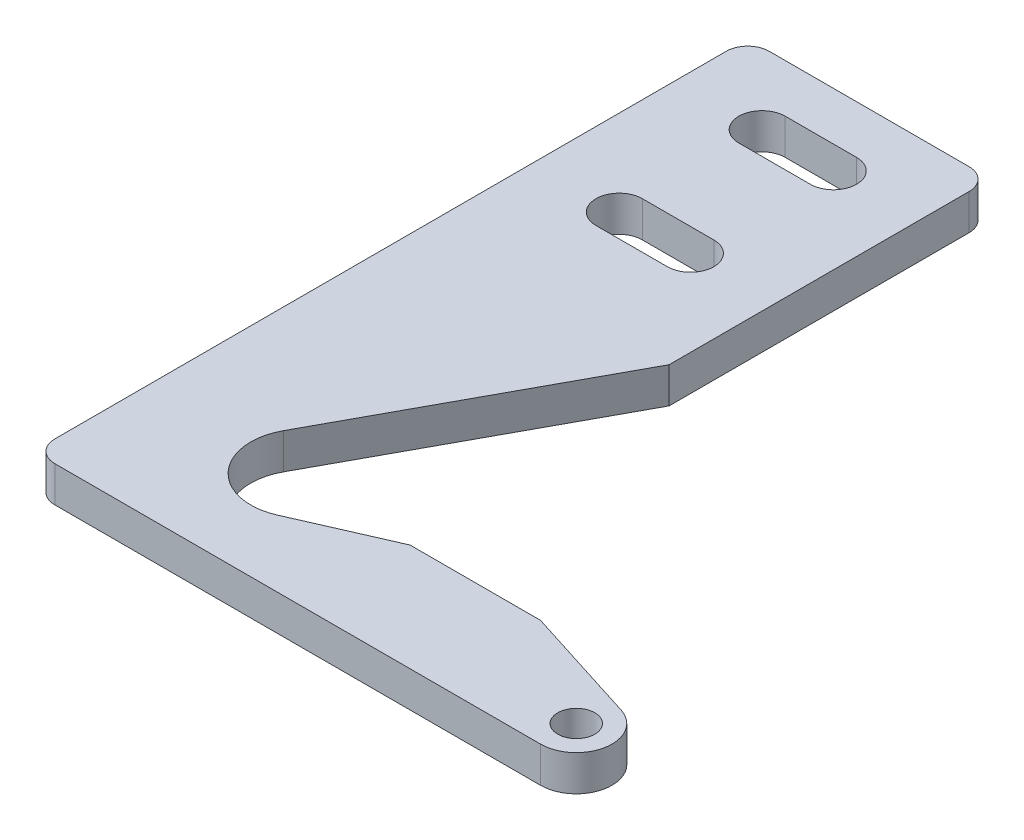
SolidWorks part; units mm, degrees
material "SPCC"
ref_plane "Front Plane" through (0, 0, 0) normal (0, 0, 1) x (1, 0, 0)
ref_plane "Top Plane" through (0, 0, 0) normal (0, 1, 0) x (1, 0, 0)
ref_plane "Right Plane" through (0, 0, 0) normal (1, 0, 0) x (0, 0, -1)
sketch "Sketch1" plane through (0, 0, 0) normal (0, 1, 0) x (1, 0, 0)
  line L0 (5, 0) -> (-5, 0) construction
  line L1 (5, -3.25) -> (-5, -3.25)
  line L2 (5, 3.25) -> (-5, 3.25)
  line L3 (5, -20) -> (-5, -20) construction
  line L4 (5, -23.25) -> (-5, -23.25)
  line L5 (5, -16.75) -> (-5, -16.75)
  line L6 (0, 0) -> (0, -20) construction
  line L7 (-17, 10) -> (-17, -90)
  line L8 (-17, 10) -> (17, 10)
  line L10 (-17, -90) -> (54, -90)
  line L12 (39, -75) -> (20.7261, -75)
  line L13 (39, -75) -> (55.5108, -80.2337)
  line L14 (17, 10) -> (17, -35)
  line L15 (17, -35) -> (-2, -70)
  line L16 (20.7261, -75) -> (7.7959, -80.6619)
  line L20 (0, -20) -> (0, -3.25) construction
  arc A0 (5, -3.25) -> (5, 3.25) centre (5, 0) ccw
  arc A1 (-5, 3.25) -> (-5, -3.25) centre (-5, 0) ccw
  arc A2 (5, -23.25) -> (5, -16.75) centre (5, -20) ccw
  arc A3 (-5, -16.75) -> (-5, -23.25) centre (-5, -20) ccw
  circle A4 centre (54, -85) radius 2.6
  arc A5 (54, -90) -> (55.5108, -80.2337) centre (54, -85) ccw
  arc A6 (-2, -70) -> (7.7959, -80.6619) centre (4.7261, -73.6513) ccw
  point P2 (0, 0)
  point P10 (0, -20)
  dimension "D10" = 5.2
  dimension "D13" = 17
  dimension "D7" = 10
  dimension "D20" = 100
  dimension "D14" = 7.6533
  dimension "D1" = 6.5
  dimension "D2" = 10
  dimension "D3" = 20
  dimension "D4" = 17
  dimension "D5" = 45
  dimension "D6" = 10
  dimension "D8" = 15
  dimension "D9" = 15
  dimension "D11" = 85
  dimension "D12" = 54
  dimension "D15" = 20
  dimension "D16" = 70
  dimension "D17" = 73.6513
  dimension "D18" = 16
extrude "Boss-Extrude1" add sketch "Sketch1" along normal blind 5
fillet "Fillet1" radius 3 3 edges at (-17, 2.5, -10) (17, 2.5, -10) (-17, 2.5, 90)
